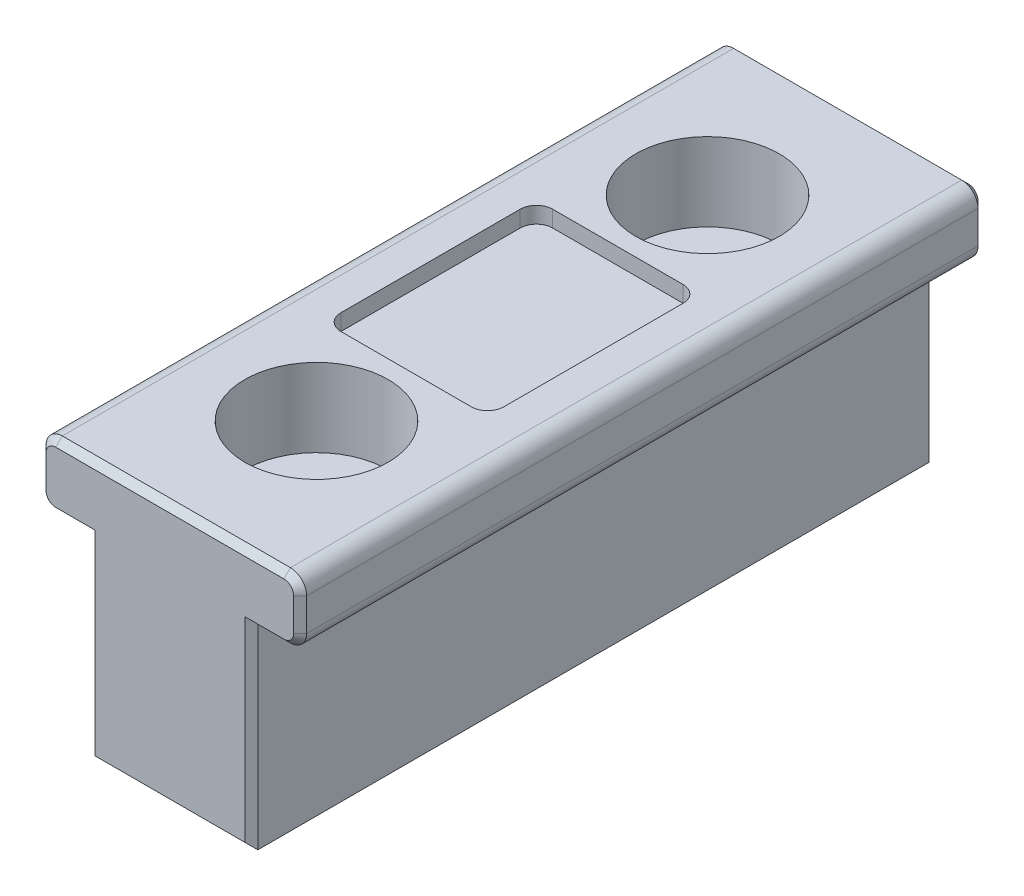
SolidWorks part; units mm, degrees
material "S136H"
ref_plane "Front Plane" through (0, 0, 0) normal (0, 0, 1) x (1, 0, 0)
ref_plane "Top Plane" through (0, 0, 0) normal (0, 1, 0) x (1, 0, 0)
ref_plane "Right Plane" through (0, 0, 0) normal (1, 0, 0) x (0, 0, -1)
sketch "Sketch1" plane through (0, 0, 0) normal (0, 0, 1) x (1, 0, 0)
  line L1 (-4, 4) -> (4, 4)
  line L2 (-4, 4) -> (-4, -4)
  line L3 (-4, -4) -> (4, -4)
  line L4 (4, 4) -> (4, -4)
  line L5 (-4, 4) -> (4, -4) construction
  line L6 (-4, -4) -> (4, 4) construction
  point P0 (0, 0)
  dimension "D1" = 8
  dimension "D2" = 8
extrude "Boss-Extrude1" add sketch "Sketch1" along normal blind 21
sketch "Sketch2" plane through (0, 0, 21) normal (0, 0, 1) x (1, 0, 0)
  line L1 (-4, -4) -> (-2.5, -4)
  line L2 (-4, -4) -> (-4, 2)
  line L3 (-4, 2) -> (-2.5, 2)
  line L4 (-2.5, -4) -> (-2.5, 2)
  line L5 (4, -4) -> (2.5, -4)
  line L6 (4, -4) -> (4, 2)
  line L7 (4, 2) -> (2.5, 2)
  line L8 (2.5, -4) -> (2.5, 2)
  dimension "D1" = 1.5
  dimension "D2" = 1.5
  dimension "D3" = 6
  dimension "D4" = 6
extrude "Cut-Extrude1" cut sketch "Sketch2" against normal through all
fillet "Fillet1" radius 0.5 4 edges at (4, 4, 10.5) (4, 2, 10.5) (-4, 4, 10.5) (-4, 2, 10.5)
hole_wizard "CBORE for M2 Hex Socket Head Cap Screw1" positions "Sketch6" profile "Sketch5" counterbore size "M2" standard "ISO" end condition through all
sketch "Sketch6" plane through (0, 4, 0) normal (0, 1, 0) x (1, 0, 0)
  line L0 (3.5, 0) -> (-3.5, 0) construction
  line L1 (3.5, -21) -> (-3.5, -21) construction
  point P0 (0, -4.5)
  point P2 (0, -16.5)
  dimension "D1" = 4.5
  dimension "D2" = 4.5
sketch "Sketch5" plane through (0, 4, 4.5) normal (1, 0, 0) x (0, 0, 1)
  line L0 (0, 0) -> (0, 8)
  line L1 (0, 8) -> (1.2, 8)
  line L3 (1.2, 8) -> (1.2, 2.4)
  line L4 (1.2, 2.4) -> (2.2, 2.4)
  line L5 (2.2, 2.4) -> (2.2, 0)
  line L7 (2.2, 0) -> (0, 0)
  line L11 (0, -6.35) -> (0, 107.95) construction
  dimension "通孔孔直径" = 2.4
  dimension "通孔孔深度" = 8
  dimension "柱形沉头孔直径" = 4.4
  dimension "柱形沉头孔深度" = 2.4
chamfer "Chamfer1" distance 0.2 angle 45 24 edges at (-3.8536, 3.8536, 0) (-4, 3, 0) (-3.8536, 2.1464, 0) (-3, 2, 0) (-2.5, -1, 0) (0, -4, 0) (2.5, -1, 0) (3, 2, 0) (3.8536, 2.1464, 0) (4, 3, 0) (3.8536, 3.8536, 0) (0, 4, 0) (3.8536, 2.1464, 21) (3, 2, 21) (2.5, -1, 21) (0, -4, 21) (-2.5, -1, 21) (-3, 2, 21) (-3.8536, 2.1464, 21) (-4, 3, 21) (-3.8536, 3.8536, 21) (0, 4, 21) (3.8536, 3.8536, 21) (4, 3, 21)
sketch "Sketch7" plane through (0, 4, 0) normal (0, 1, 0) x (1, 0, 0)
  line L0 (0, -0.2) -> (0, -20.8) construction
  line L1 (3.5, -0.2) -> (-3.5, -0.2) construction
  line L2 (-3.5, -20.8) -> (3.5, -20.8) construction
  line L4 (-2.5, -13.75) -> (2.5, -13.75)
  line L5 (-2.5, -13.75) -> (-2.5, -7.25)
  line L6 (-2.5, -7.25) -> (2.5, -7.25)
  line L7 (2.5, -13.75) -> (2.5, -7.25)
  line L8 (-2.5, -13.75) -> (2.5, -7.25) construction
  line L9 (-2.5, -7.25) -> (2.5, -13.75) construction
  point P6 (0, -10.5)
  dimension "D1" = 5
  dimension "D2" = 6.5
extrude "Cut-Extrude2" cut sketch "Sketch7" against normal blind 0.5
fillet "Fillet2" radius 0.5 4 edges at (-2.5, 3.75, 13.75) (2.5, 3.75, 13.75) (2.5, 3.75, 7.25) (-2.5, 3.75, 7.25)
equation "\"code1\"= \"图名分离代码\""
equation "\"code2\"= \"图号分离代码\""
